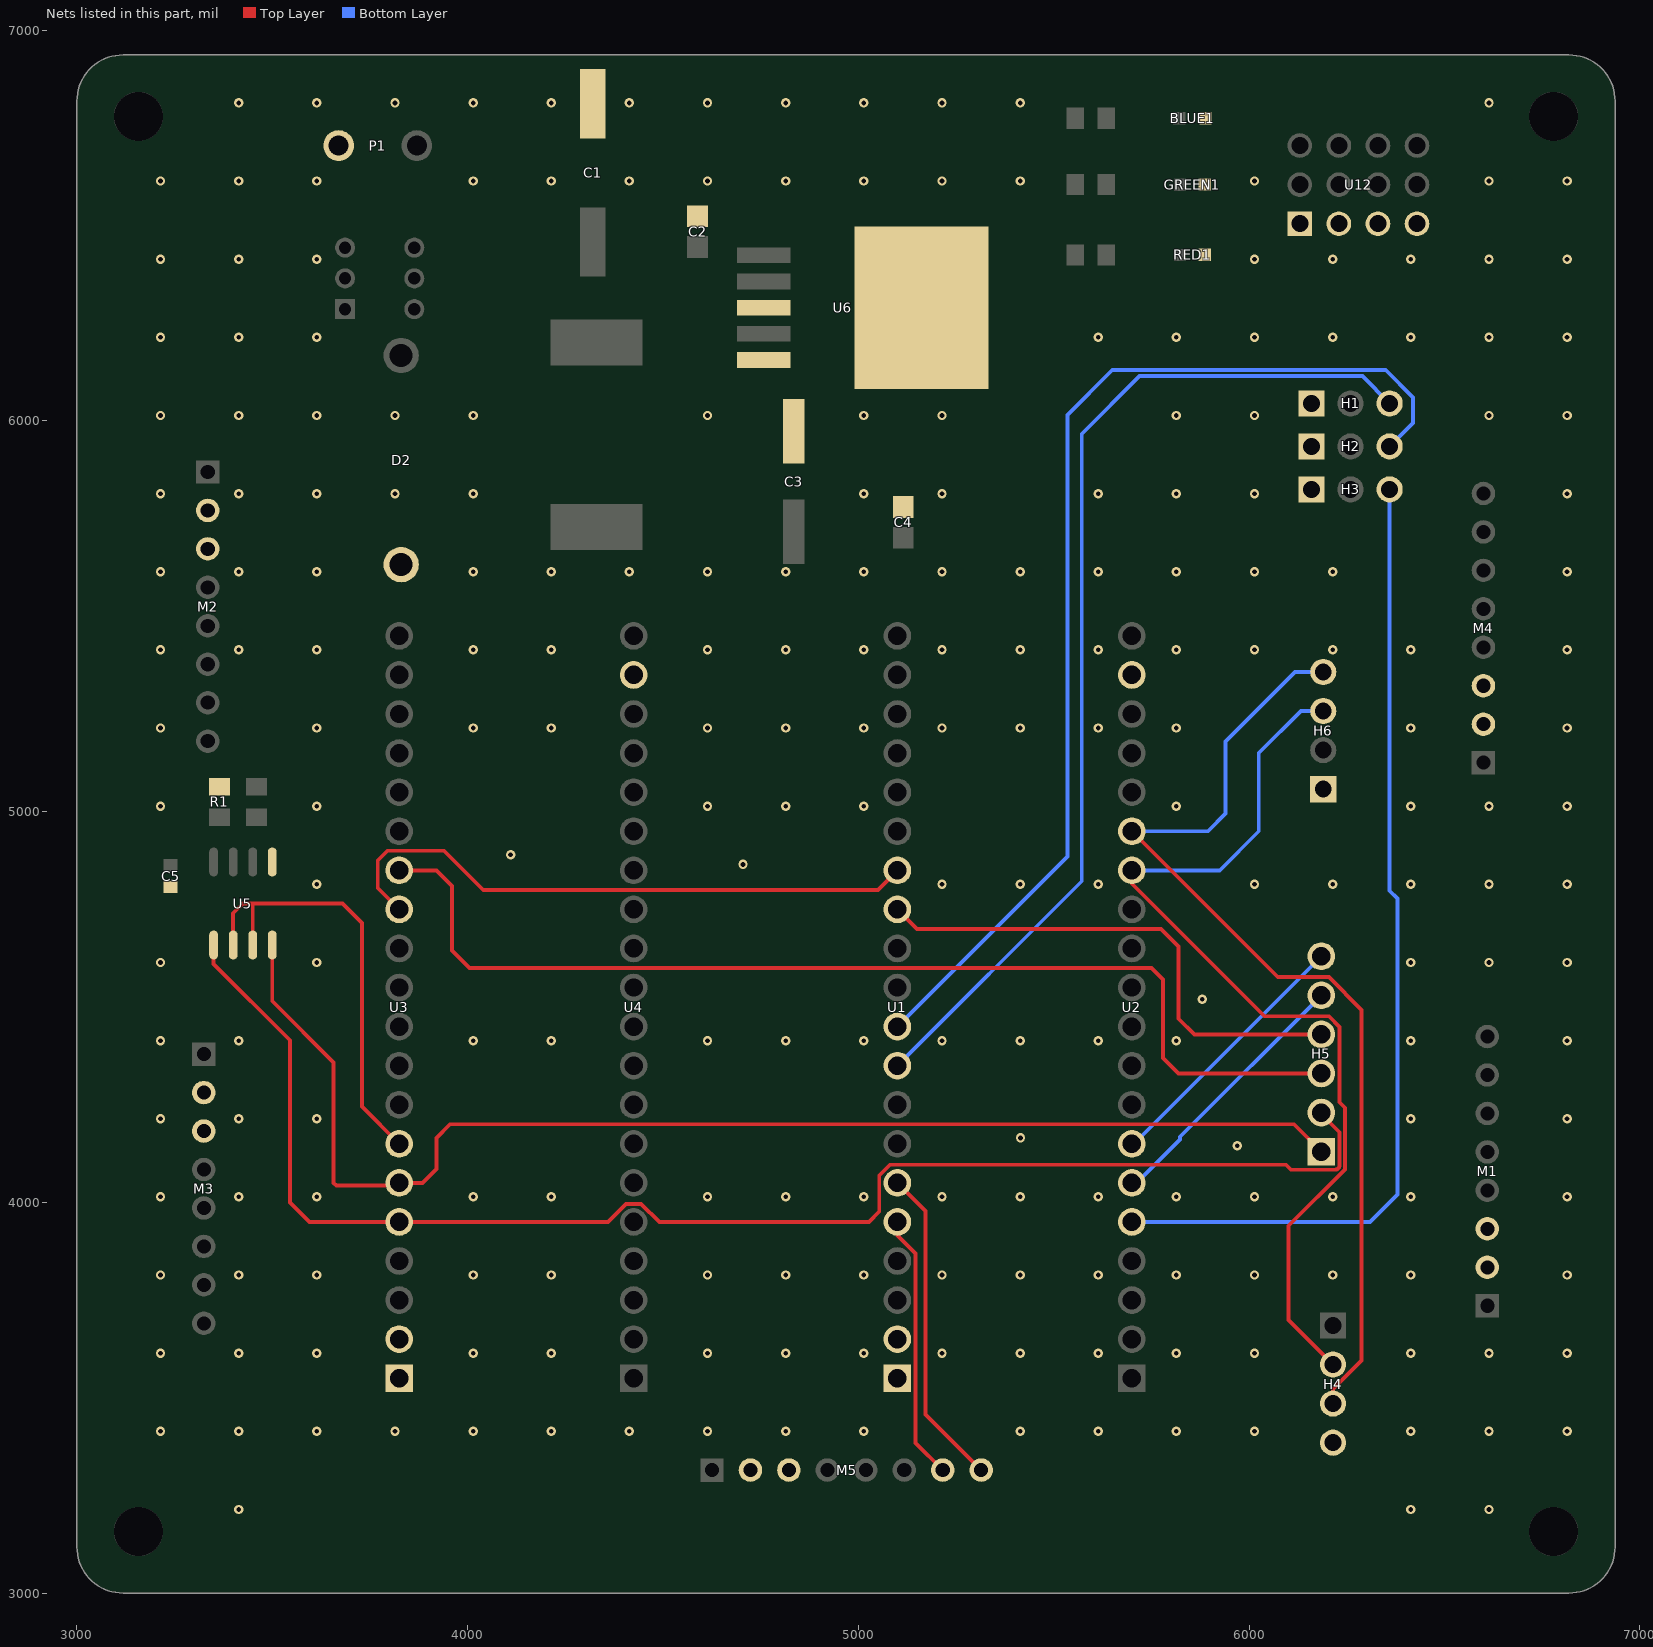
[diagram p0: the nets of this part, all layers, seen from the top]
# Altium PCB MISC50151.pcbdoc (part 2 of 4)
Units mil, origin at the board's own origin, x right, y up, seen from the top; angles counter-clockwise.
Board outline 3937.01 x 3937.01 mil, 4 copper layers (Top Layer, Inner1, Inner2, Bottom Layer), stack 62.447 mil thick; 39 components, 26 nets, 211 pads, 230 vias.

## Via types
v1: diameter 24.02, hole 12, Top Layer to Bottom Layer, 230 vias

## Nets (pads, with @x,y where several pads share a name; then routed paths per layer and width w, separated by ;. In a path a pad name is that pad's centre, name@x,y a point inside that pad or via, vN(x,y) a via of type N, cw(c..) or ccw(c..) an arc to the next point about the centre after c; other vN are vias at no path point) (continued)
GND: BLUE1.2 C1.2 C2.1 C3.2 C4.1 C5.2 D2.2 GREEN1.1 H1.1 H2.1 H3.1 H4.4 H6.1 M1.2 M1.3 M2.2 M2.3 M3.2 M3.3 M4.2 M4.3 M5.2 M5.3 P1.1 R1.2 RED1.1 U1.1 U1.2 U2.19 U3.1 U3.2 U4.19 U5.5 U6.3 U6.5 U6.6 U12.1 U12.4 U12.7 U12.10
  other v1: 3414.1,3214.1 6414.1,3214.1 6614.1,3214.1 3214.1,3414.1 3414.1,3414.1 3614.1,3414.1 3814.1,3414.1 4014.1,3414.1 4214.1,3414.1 4414.1,3414.1 4614.1,3414.1 4814.1,3414.1 5014.1,3414.1 5414.1,3414.1 5614.1,3414.1 5814.1,3414.1 6014.1,3414.1 6414.1,3414.1 6614.1,3414.1 6814.1,3414.1 3214.1,3614.1 3414.1,3614.1 3614.1,3614.1 4014.1,3614.1 4214.1,3614.1 4614.1,3614.1 4814.1,3614.1 5014.1,3614.1 5214.1,3614.1 5414.1,3614.1 5614.1,3614.1 5814.1,3614.1 6014.1,3614.1 6414.1,3614.1 6614.1,3614.1 6814.1,3614.1 3214.1,3814.1 3414.1,3814.1 3614.1,3814.1 4014.1,3814.1 4214.1,3814.1 4614.1,3814.1 4814.1,3814.1 5014.1,3814.1 5214.1,3814.1 5414.1,3814.1 5614.1,3814.1 5814.1,3814.1 6014.1,3814.1 6214.1,3814.1 6414.1,3814.1 6814.1,3814.1 3214.1,4014.1 3414.1,4014.1 3614.1,4014.1 4014.1,4014.1 4214.1,4014.1 4614.1,4014.1 4814.1,4014.1 5014.1,4014.1 5214.1,4014.1 5414.1,4014.1 5614.1,4014.1 5814.1,4014.1 6014.1,4014.1 6214.1,4014.1 6414.1,4014.1 6814.1,4014.1 5970,4145 5415,4165 3214.1,4214.1 3414.1,4214.1 3614.1,4214.1 6414.1,4214.1 6814.1,4214.1 3214.1,4414.1 3414.1,4414.1 4014.1,4414.1 4214.1,4414.1 4614.1,4414.1 4814.1,4414.1 5014.1,4414.1 5214.1,4414.1 5414.1,4414.1 5614.1,4414.1 5814.1,4414.1 6414.1,4414.1 6814.1,4414.1 5880,4520 3214.1,4614.1 3614.1,4614.1 6414.1,4614.1 6614.1,4614.1 6814.1,4614.1 3614.1,4814.1 5214.1,4814.1 5414.1,4814.1 5614.1,4814.1 6014.1,4814.1 6214.1,4814.1 6414.1,4814.1 6614.1,4814.1 6814.1,4814.1 4705,4865 4110,4890 3214.1,5014.1 3614.1,5014.1 4614.1,5014.1 4814.1,5014.1 5014.1,5014.1 5814.1,5014.1 6414.1,5014.1 6614.1,5014.1 6814.1,5014.1 3214.1,5214.1 3614.1,5214.1 4014.1,5214.1 4214.1,5214.1 4614.1,5214.1 4814.1,5214.1 5014.1,5214.1 5214.1,5214.1 5414.1,5214.1 5614.1,5214.1 5814.1,5214.1 6414.1,5214.1 6814.1,5214.1 3214.1,5414.1 3414.1,5414.1 3614.1,5414.1 4014.1,5414.1 4214.1,5414.1 4614.1,5414.1 4814.1,5414.1 5014.1,5414.1 5214.1,5414.1 5414.1,5414.1 5614.1,5414.1 5814.1,5414.1 6014.1,5414.1 6214.1,5414.1 6414.1,5414.1 6814.1,5414.1 3214.1,5614.1 3414.1,5614.1 3614.1,5614.1 4014.1,5614.1 4214.1,5614.1 4414.1,5614.1 4614.1,5614.1 4814.1,5614.1 5014.1,5614.1 5214.1,5614.1 5414.1,5614.1 5614.1,5614.1 5814.1,5614.1 6014.1,5614.1 6214.1,5614.1 6814.1,5614.1 3214.1,5814.1 3414.1,5814.1 3614.1,5814.1 3814.1,5814.1 4014.1,5814.1 5014.1,5814.1 5214.1,5814.1 5614.1,5814.1 5814.1,5814.1 6014.1,5814.1 6814.1,5814.1 3214.1,6014.1 3414.1,6014.1 3614.1,6014.1 3814.1,6014.1 4014.1,6014.1 4614.1,6014.1 5014.1,6014.1 5214.1,6014.1 5814.1,6014.1 6014.1,6014.1 6614.1,6014.1 6814.1,6014.1 3214.1,6214.1 3414.1,6214.1 3614.1,6214.1 5614.1,6214.1 5814.1,6214.1 6014.1,6214.1 6214.1,6214.1 6414.1,6214.1 6614.1,6214.1 6814.1,6214.1 3214.1,6414.1 3414.1,6414.1 3614.1,6414.1 6014.1,6414.1 6214.1,6414.1 6414.1,6414.1 6614.1,6414.1 6814.1,6414.1 3214.1,6614.1 3414.1,6614.1 3614.1,6614.1 4014.1,6614.1 4214.1,6614.1 4414.1,6614.1 4614.1,6614.1 4814.1,6614.1 5014.1,6614.1 5214.1,6614.1 5414.1,6614.1 6014.1,6614.1 6614.1,6614.1 6814.1,6614.1 3414.1,6814.1 3614.1,6814.1 3814.1,6814.1 4014.1,6814.1 4214.1,6814.1 4414.1,6814.1 4614.1,6814.1 4814.1,6814.1 5014.1,6814.1 5214.1,6814.1 5414.1,6814.1 6614.1,6814.1
M_GYRO_SCL: H4.2 H6.3 U2.14 | length 2470.2
  Top Layer w10: U2.14@5700,4850 5700,4815.64 6039.23,4476.42 6204.23,4476.42 6231.42,4449.23 6231.42,4256.39 6245.43,4242.38 6245.43,4084.21 6101.48,3940.26 6101.48,3698.52 H4.2@6215,3585
  Bottom Layer w10: U2.14@5700,4850 5925,4850 6025,4950 6025,5150 6132.57,5257.57 H6.3@6190,5257.57
M_GYRO_SDA: H4.3 H6.4 U2.15 | length 2582.5
  Top Layer w10: U2.15@5700,4950 6073.58,4576.42 6204.23,4576.42 6287.99,4492.65 6287.99,3595.13 6215,3522.14 H4.3@6215,3485
  Bottom Layer w10: U2.15@5700,4950 5895,4950 5940,4995 5940,5180 6117.57,5357.57 H6.4@6190,5357.57
M_MASTER_RX: H5.6 U2.7 | length 683.8
  Bottom Layer w10: U2.7@5700,4150 5705,4150 H5.6@6185,4630
M_MASTER_TX: H5.5 U2.6 | length 688.2
  Bottom Layer w10: U2.6@5700,4050 5712.52,4050 5822.99,4160.48 5822.99,4167.99 H5.5@6185,4530
M_MOTER5_RX: M5.7 U1.5 | length 683.1
  Top Layer w10: U1.5@5100,3950 5100,3915.64 5146.42,3869.23 5146.42,3384.64 M5.7@5216.06,3315
M_MOTER5_TX: M5.8 U1.6 | length 823.8
  Top Layer w10: U1.6@5100,4050 5172.01,3977.99 5172.01,3457.48 M5.8@5314.48,3315
M_PWM1: H1.3 U1.9 | length 2690.8
  Bottom Layer w10: U1.9@5100,4350 5572.01,4822.01 5572.01,5967.01 5720,6115 6290,6115 H1.3@6360,6045
M_PWM2: H2.3 U1.10 | length 2856.7
  Bottom Layer w10: U1.10@5100,4450 5535,4885 5535,6015 5650,6130 6350,6130 6420,6060 6420,5995 H2.3@6360,5935
M_PWM3: H3.3 U2.5 | length 2522.3
  Bottom Layer w10: U2.5@5700,3950 6310,3950 6380,4020 6380,4777.71 6360,4797.71 H3.3@6360,5825
M_SAVE_RX: H5.4 U1.13 | length 1325.9
  Top Layer w10: U1.13@5100,4750 5150,4700 5775,4700 5820,4655 5820,4470 5860,4430 H5.4@6185,4430
M_SLAVE_TX: U1.14 U3.13 | length 1550.3
  Top Layer w10: U3.13@3825,4750 3770,4805 3770,4875 3795,4900 3940,4900 4040,4800 5050,4800 U1.14@5100,4850
S_485_EN: U3.7 U5.2 U5.3 | length 1152.9
  Top Layer w10: U5.2@3400,4658.74 3400,4740 3425,4765 3450,4765 ; U5.3@3450,4658.74 3450,4765 ; U3.7@3825,4150 3730,4245 3730,4715 3680,4765 3450,4765
S_SAVE_2_TX: H5.3 U3.14 | length 2789.2
  Top Layer w10: U3.14@3825,4850 3920,4850 3960,4810 3960,4645 4005,4600 5750,4600 5780,4570 5780,4370 5820,4330 H5.3@6185,4330
S_SAVE_3_RX: H5.2 U3.5 U5.1 | length 3766.4
  Top Layer w10: U5.1@3350,4658.74 3350,4610 3545,4415 3545,4000 3595,3950 U3.5@3825,3950 4359.36,3950 4405.77,3996.42 4444.23,3996.42 4490.64,3950 5027.19,3950 5053.58,3976.39 5053.58,4069.23 5080.77,4096.42 6094.45,4096.42 6107.29,4083.58 6220.43,4083.58 ccw(c6220.43,4094.57) 6231.42,4094.57 6231.42,4179.47 6185,4225.89 H5.2@6185,4230
S_SAVE_3_TX: H5.1 U3.6 U5.4 | length 3345.6
  Top Layer w10: U5.4@3500,4658.74 3500,4515 3657.07,4357.93 3657.07,4050 3664.14,4042.93 3817.93,4042.93 U3.6@3825,4050 3885,4050 3920,4085 3920,4165 3955,4200 6115,4200 H5.1@6185,4130
pads on no net: M1.4 M1.5 M1.6 M2.4 M2.5 M2.6 M3.4 M3.5 M3.6 M4.4 M4.5 M4.6 M5.4 M5.5 M5.6 SCREW1.1 SCREW2.1 SCREW3.1 SCREW4.1 SW1.1 SW1.2 SW1.3 SW1.4 U1.4 U1.7 U1.8 U1.11 U1.12 U1.15 U1.16 U1.17 U1.18 U1.19 U1.20 U2.1 U2.2 U2.3 U2.4 U2.8 U2.9 U2.10 U2.11 U2.12 U2.13 U2.16 U2.17 U2.18 U3.4 U3.8 U3.9 U3.10 U3.11 U3.12 U3.15 U3.16 U3.17 U3.18 U3.19 U3.20 U4.1 U4.2 U4.3 U4.4 U4.5 U4.6 U4.7 U4.8 U4.9 U4.10 U4.11 U4.12 U4.13 U4.14 U4.15 U4.16 U4.17 U4.18

## Polygon pours and split planes (outlines as drawn)
GND on Top Layer (solid, remove dead copper, pour order 0): 3118.11,6937.01 ccw(c3118.11,6818.9) 3000,6818.9 3000,3118.11 ccw(c3118.11,3118.11) 3118.11,3000 6818.9,3000 ccw(c6818.9,3118.11) 6937.01,3118.11 6937.01,6818.9 ccw(c6818.9,6818.9) 6818.9,6937.01 3118.11,6937.01
GND on Inner2 (solid, remove dead copper): 3118.11,6937.01 ccw(c3118.11,6818.9) 3000,6818.9 3000,3118.11 ccw(c3118.11,3118.11) 3118.11,3000 6818.9,3000 ccw(c6818.9,3118.11) 6937.01,3118.11 6937.01,6818.9 ccw(c6818.9,6818.9) 6818.9,6937.01 3118.11,6937.01
GND on Inner1 (solid, remove dead copper): 3118.11,6937.01 ccw(c3118.11,6818.9) 3000,6818.9 3000,3118.11 ccw(c3118.11,3118.11) 3118.11,3000 6818.9,3000 ccw(c6818.9,3118.11) 6937.01,3118.11 6937.01,6818.9 ccw(c6818.9,6818.9) 6818.9,6937.01 3118.11,6937.01
GND on Bottom Layer (solid, remove dead copper, pour order 2): 3118.11,6937.01 ccw(c3118.11,6818.9) 3000,6818.9 3000,3118.11 ccw(c3118.11,3118.11) 3118.11,3000 6818.9,3000 ccw(c6818.9,3118.11) 6937.01,3118.11 6937.01,6818.9 ccw(c6818.9,6818.9) 6818.9,6937.01 3118.11,6937.01

## Keep-outs
Board Outline Layer:
  the board outline again, w10